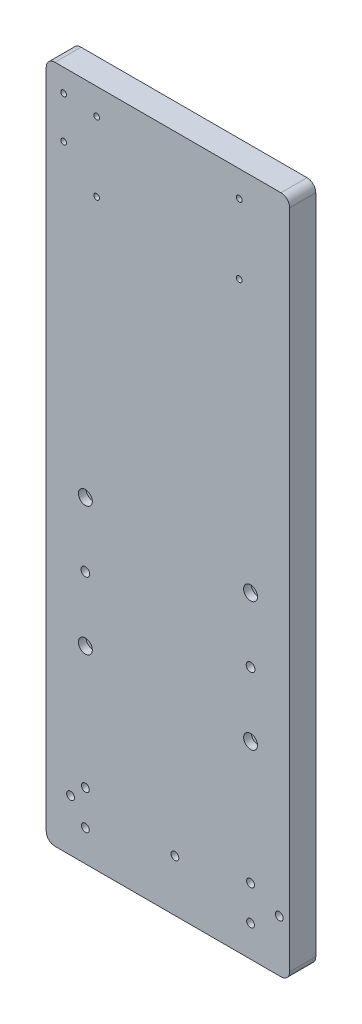
from build123d import *

# Parameters (mm, degrees)
SKETCH_1_W                   = 140
SKETCH_1_H                   = 390.5
EXTRUDE_1_DEPTH              = 15
HOLE_WIZARD_M5_6_D           = 4.5
HOLE_WIZARD_M5_6_CBORE_D     = 8
HOLE_WIZARD_M5_6_CBORE_DEPTH = 4.4
HOLE_WIZARD_5_0_5_1_D        = 5
FILLET_1_R                   = 5
HOLE_WIZARD_M4_3_D           = 3.3
HOLE_WIZARD_M4_1_D           = 4.5
HOLE_WIZARD_M4_1_CBORE_D     = 8
HOLE_WIZARD_M4_1_CBORE_DEPTH = 4.4
HOLE_WIZARD_M4_6_D           = 3.3
HOLE_WIZARD_M4_6_DEPTH       = 15
HOLE_WIZARD_M4_6_TIP         = 0.991420021
HOLE_WIZARD_M4_7_D           = 3.3
HOLE_WIZARD_M4_2_D           = 4.5
HOLE_WIZARD_M4_2_CBORE_D     = 8
HOLE_WIZARD_M4_2_CBORE_DEPTH = 4.4


with BuildPart() as part:
    # 草图1 → 凸台-拉伸1 (new body)
    with BuildSketch(Plane.XY):
        Rectangle(SKETCH_1_W, SKETCH_1_H)
    extrude(amount=EXTRUDE_1_DEPTH)

    # M5 六角凹头螺钉的柱形沉头孔6 (through all)
    with Locations(Plane.XY.offset(15)):
        with Locations((-47.5, -12.75), (-47.5, -86.75), (47.5, -12.75), (47.5, -86.75)):
            CounterBoreHole(HOLE_WIZARD_M5_6_D / 2, HOLE_WIZARD_M5_6_CBORE_D / 2, HOLE_WIZARD_M5_6_CBORE_DEPTH)

    # Ø5.0 (5) 直径孔1 (through all)
    with Locations(Plane.XY.offset(15)):
        with Locations((-47.5, -49.75), (47.5, -49.75)):
            Hole(HOLE_WIZARD_5_0_5_1_D / 2)

    # 圆角1
    fillet_1_edges = [part.edges().sort_by_distance(p)[0] for p in [
        (70, -195.25, 7.5),
        (-70, -195.25, 7.5),
        (-70, 195.25, 7.5),
        (70, 195.25, 7.5),
    ]]
    fillet(fillet_1_edges, radius=FILLET_1_R)

    # M4 螺纹孔3 (through all)
    with Locations(Plane.XY.offset(15)):
        with Locations((-41, 180.25), (41, 180.25), (41, 140.25), (-41, 140.25)):
            Hole(HOLE_WIZARD_M4_3_D / 2)

    # M4 六角凹头螺钉的柱形沉头孔1 (through all)
    with Locations(Plane(origin=(0, 0, 0), x_dir=(-1, 0, 0), z_dir=(0, 0, -1))):
        with Locations((47.5, -157.25), (47.5, -177.25), (-47.5, -157.25), (-47.5, -177.25)):
            CounterBoreHole(HOLE_WIZARD_M4_1_D / 2, HOLE_WIZARD_M4_1_CBORE_D / 2, HOLE_WIZARD_M4_1_CBORE_DEPTH)

    # M4 螺纹孔6
    with Locations(Plane.ZY.offset(70)):
        with Locations((7.5, 185.25), (7.5, 170.25), (7.5, 155.25)):
            Hole(HOLE_WIZARD_M4_6_D / 2, depth=HOLE_WIZARD_M4_6_DEPTH)
            with Locations((0, 0, -(HOLE_WIZARD_M4_6_DEPTH + HOLE_WIZARD_M4_6_TIP / 2))):  # 118° drill point
                Cone(0, HOLE_WIZARD_M4_6_D / 2, HOLE_WIZARD_M4_6_TIP, mode=Mode.SUBTRACT)

    # M4 螺纹孔7 (through all)
    with Locations(Plane.XY.offset(15)):
        with Locations((-60, 182.25), (-60, 158.25)):
            Hole(HOLE_WIZARD_M4_7_D / 2)

    # M4 六角凹头螺钉的柱形沉头孔2 (through all)
    with Locations(Plane(origin=(0, 0, 0), x_dir=(-1, 0, 0), z_dir=(0, 0, -1))):
        with Locations((-64, -165.54), (-4, -165.54), (-64, -225.54), (-4, -225.54), (56, -165.54), (56, -225.54)):
            CounterBoreHole(HOLE_WIZARD_M4_2_D / 2, HOLE_WIZARD_M4_2_CBORE_D / 2, HOLE_WIZARD_M4_2_CBORE_DEPTH)


solid = part.part
